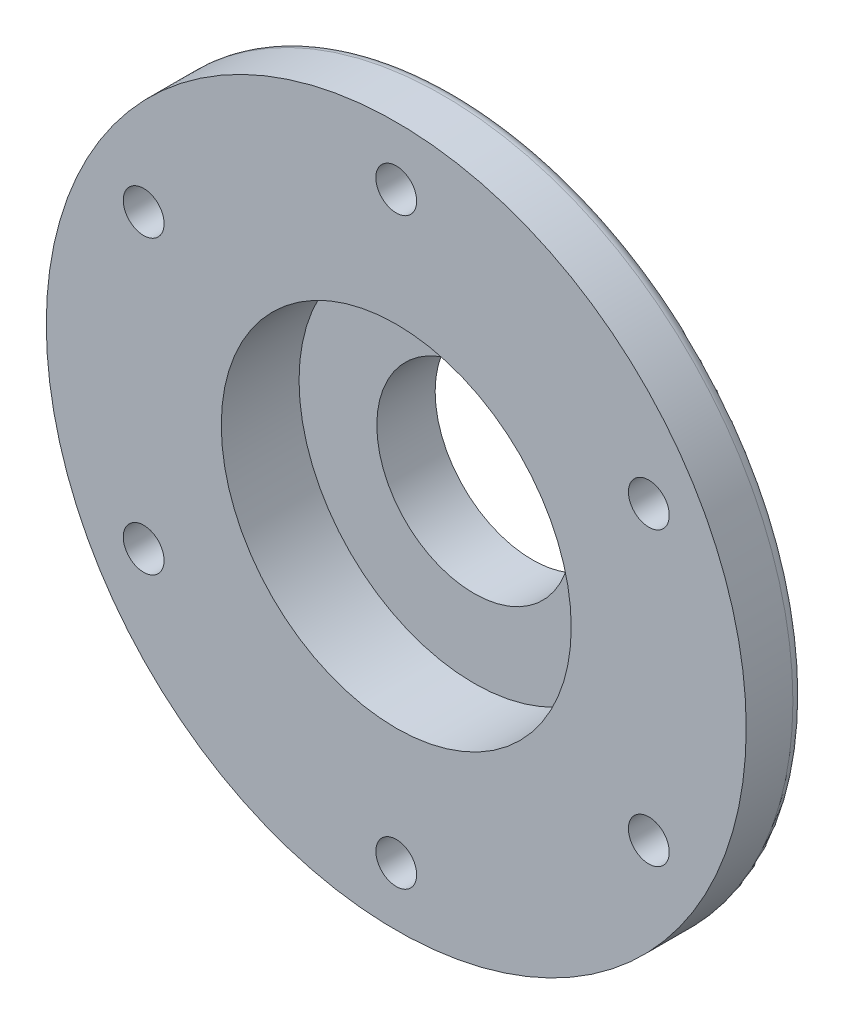
SolidWorks part; units mm, degrees
material "普通碳钢"
ref_plane "前视基准面" through (0, 0, 0) normal (0, 0, 1) x (1, 0, 0)
ref_plane "上视基准面" through (0, 0, 0) normal (0, 1, 0) x (1, 0, 0)
ref_plane "右视基准面" through (0, 0, 0) normal (1, 0, 0) x (0, 0, -1)
sketch "草图1" plane through (0, 0, 0) normal (0, 0, 1) x (1, 0, 0)
  line L0 (0, 0) -> (0, 77.0152) construction
  circle A0 centre (0, 0) radius 90
  circle A1 centre (0, 0) radius 25
  circle A2 centre (0, 75) radius 5.25
  circle A3 centre (64.9519, 37.5) radius 5.25
  circle A4 centre (64.9519, -37.5) radius 5.25
  circle A5 centre (0, -75) radius 5.25
  circle A6 centre (-64.9519, -37.5) radius 5.25
  circle A7 centre (-64.9519, 37.5) radius 5.25
  point P20 (0, 0)
  dimension "D1" = 180
  dimension "D2" = 50
  dimension "D3" = 10.5
  dimension "D4" = 75
  dimension "D5" = 6
extrude "凸台-拉伸1" add sketch "草图1" along normal blind 15
sketch "草图2" plane through (0, 0, 0) normal (0, 0, -1) x (-1, 0, 0)
  circle A0 centre (0, 0) radius 55
  circle A1 centre (0, 0) radius 25 construction
  circle A2 centre (0, 0) radius 25
  dimension "D1" = 110
extrude "凸台-拉伸2" add sketch "草图2" along normal blind 20
sketch "草图3" plane through (0, 0, 15) normal (0, 0, 1) x (1, 0, 0)
  circle A0 centre (0, 0) radius 45
  dimension "D1" = 90
extrude "切除-拉伸1" cut sketch "草图3" against normal blind 20
fillet "圆角1" radius 3 3 edges at (55, 0, 0) (90, 0, 0) (-55, 0, -20)
